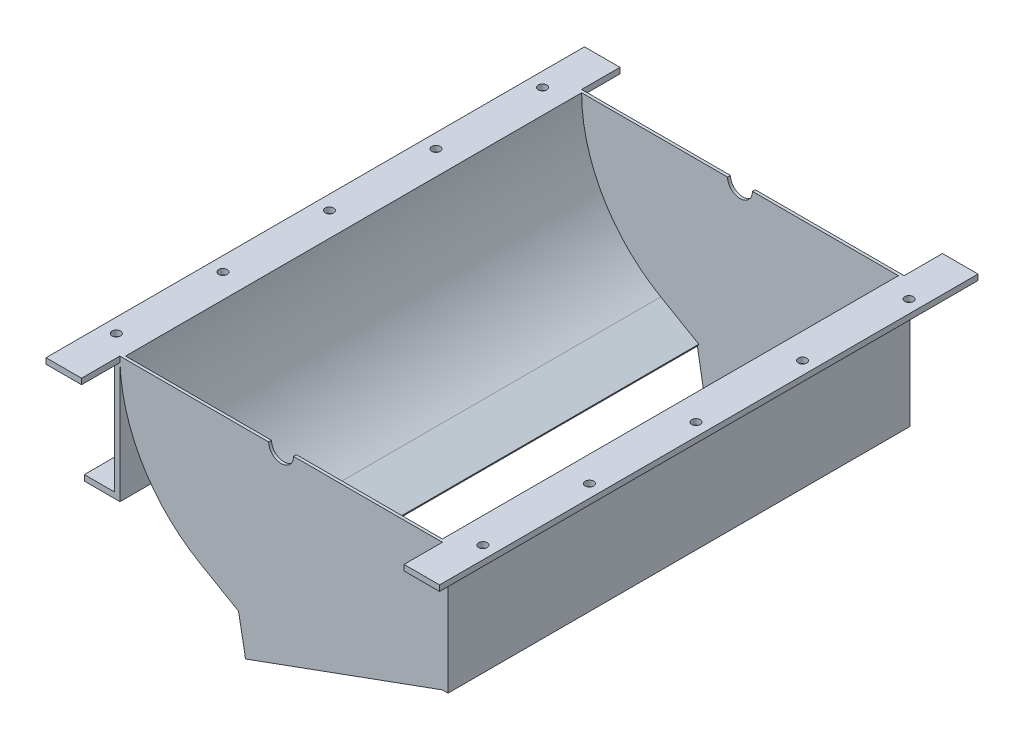
SolidWorks part; units mm, degrees
material "AISI 304"
ref_plane "Front Plane" through (0, 0, 0) normal (0, 0, 1) x (1, 0, 0)
ref_plane "Top Plane" through (0, 0, 0) normal (0, 1, 0) x (1, 0, 0)
ref_plane "Right Plane" through (0, 0, 0) normal (1, 0, 0) x (0, 0, -1)
other "Configuration Table"
sketch "Sketch1" plane through (0, 0, 0) normal (0, 0, 1) x (1, 0, 0)
  line L0 (-227, 0) -> (-227, 377)
  line L1 (-227, 377) -> (0, 377)
  line L2 (0, 377) -> (0, 227)
  line L3 (-223, 0) -> (-223, 377)
  line L4 (-3, 377) -> (-3, 226.9802)
  line L5 (-227, 0) -> (227, 0) construction
  line L7 (227, -180) -> (-50, -280.8198)
  line L8 (223, 0) -> (223, -177.1992)
  line L9 (223, -177.1992) -> (-51.3681, -277.061)
  line L10 (-51.3681, -277.061) -> (-50, -280.8198)
  line L11 (-113.5, -196.5878) -> (-60, -227.476)
  line L12 (-111.5, -193.1237) -> (-58, -224.0119)
  line L13 (-58, -224.0119) -> (-60, -227.476)
  line L14 (-227, 0) -> (-277, 0) construction
  line L15 (227, 0) -> (277, 0) construction
  line L16 (-50, -280.8198) -> (330.4492, -280.8198) construction
  line L17 (-277, 0) -> (-223, 0)
  line L18 (-277, 0) -> (-277, 6)
  line L19 (-277, 6) -> (-223, 6)
  line L20 (-223, 0) -> (-223, 6)
  line L21 (277, 0) -> (226.9207, 0)
  line L22 (277, 0) -> (277, 6)
  line L23 (277, 6) -> (226.9207, 6)
  line L24 (226.9207, 0) -> (226.9207, 6)
  line L25 (-277, 0) -> (-226.859, 0)
  line L26 (-277, 0) -> (-277, -8)
  line L27 (-277, -8) -> (-234.859, -8)
  line L29 (277, 0) -> (223, 0)
  line L30 (277, 0) -> (277, -8)
  line L31 (277, -8) -> (235, -8)
  line L32 (223, 0) -> (223, -8)
  line L34 (-226.859, -8) -> (-226.859, -227.476)
  line L35 (-226.859, -227.476) -> (-234.859, -227.476)
  line L36 (-234.859, -8) -> (-234.859, -219.476)
  line L38 (235, -8) -> (235, -219.476)
  line L39 (235, -227.476) -> (227, -227.476)
  line L40 (227, -180) -> (227, -227.476)
  line L41 (-60, -227.476) -> (-291.314, -227.476) construction
  line L42 (-60, -227.476) -> (-226.859, -227.476)
  line L43 (235, -227.476) -> (279, -227.476)
  line L45 (235, -219.476) -> (279, -219.476)
  line L46 (279, -227.476) -> (279, -219.476)
  line L47 (-234.859, -227.476) -> (-278.859, -227.476)
  line L49 (-234.859, -219.476) -> (-278.859, -219.476)
  line L50 (-278.859, -227.476) -> (-278.859, -219.476)
  line L51 (227, -8) -> (226.859, -8)
  line L52 (227, 0) -> (227, -180) construction
  circle A0 centre (0, 0) radius 208
  circle A1 centre (0, 0) radius 223
  arc A2 (-226.859, -8) -> (223, -42.4264) centre (0, 0) ccw
  circle A3 centre (0, 0) radius 227 construction
  arc A4 (227, 0) -> (-227, 0) centre (0, 0) ccw
  dimension "D1" = 416
  dimension "D4" = 150
  dimension "D5" = 3
  dimension "D6" = 180
  dimension "D8" = 50
  dimension "D10" = 30
  dimension "D11" = 60
  dimension "D12" = 4
  dimension "D13" = 50
  dimension "D14" = 50
  dimension "D15" = 6
  dimension "D16" = 6
  dimension "D17" = 8
  dimension "D18" = 8
  dimension "D19" = 8
  dimension "D20" = 8
  dimension "D21" = 0
  dimension "D22" = 0
  dimension "D23" = 44
  dimension "D24" = 8
  dimension "D25" = 8
  dimension "D26" = 44
  dimension "D2" = 15
  dimension "D3" = 4
  dimension "D9" = 4
extrude "Boss-Extrude2" add sketch "Sketch1" along normal mid plane 650
sketch "Sketch3" plane through (0, 0, 325) normal (0, 0, 1) x (1, 0, 0)
  line L0 (-226.859, -227.476) -> (-226.859, -8) construction
  line L1 (-113.5, -196.5878) -> (-60, -227.476) construction
  line L2 (-60, -227.476) -> (-58, -224.0119) construction
  line L3 (-58, -224.0119) -> (-111.5, -193.1237) construction
  line L4 (-223, 0) -> (-277, 0) construction
  line L5 (-277, 0) -> (-277, -8) construction
  line L6 (-277, -8) -> (-234.859, -8) construction
  line L7 (-234.859, -8) -> (-234.859, -219.476) construction
  line L8 (-234.859, -219.476) -> (-278.859, -219.476) construction
  line L9 (-278.859, -219.476) -> (-278.859, -227.476) construction
  line L10 (-278.859, -227.476) -> (-226.859, -227.476) construction
  line L11 (227, -227.476) -> (279, -227.476) construction
  line L12 (279, -227.476) -> (279, -219.476) construction
  line L13 (279, -219.476) -> (235, -219.476) construction
  line L14 (235, -219.476) -> (235, -8) construction
  line L15 (235, -8) -> (277, -8) construction
  line L16 (277, -8) -> (277, 0) construction
  line L17 (277, 0) -> (223, 0) construction
  line L18 (223, 0) -> (223, -177.1992) construction
  line L19 (223, -177.1992) -> (-51.3681, -277.061) construction
  line L20 (-51.3681, -277.061) -> (-50, -280.8198) construction
  line L21 (-50, -280.8198) -> (227, -180) construction
  line L22 (227, -180) -> (227, -227.476) construction
  line L23 (-226.859, -227.476) -> (-226.859, -8)
  line L24 (-113.5, -196.5878) -> (-60, -227.476)
  line L25 (-60, -227.476) -> (-58, -224.0119)
  line L26 (-58, -224.0119) -> (-111.5, -193.1237)
  line L27 (-223, 0) -> (-277, 0)
  line L28 (-277, 0) -> (-277, -8)
  line L29 (-277, -8) -> (-234.859, -8)
  line L30 (-234.859, -8) -> (-234.859, -219.476)
  line L31 (-234.859, -219.476) -> (-278.859, -219.476)
  line L32 (-278.859, -219.476) -> (-278.859, -227.476)
  line L33 (-278.859, -227.476) -> (-226.859, -227.476)
  line L34 (227, -227.476) -> (279, -227.476)
  line L35 (279, -227.476) -> (279, -219.476)
  line L36 (279, -219.476) -> (235, -219.476)
  line L37 (235, -219.476) -> (235, -8)
  line L38 (235, -8) -> (277, -8)
  line L39 (277, -8) -> (277, 0)
  line L40 (277, 0) -> (223, 0)
  line L41 (223, 0) -> (223, -177.1992)
  line L42 (223, -177.1992) -> (-51.3681, -277.061)
  line L43 (-51.3681, -277.061) -> (-50, -280.8198)
  line L44 (-50, -280.8198) -> (227, -180)
  line L45 (227, -180) -> (227, -227.476)
  line L46 (-60, -227.476) -> (-50, -280.8198)
  line L47 (-226.859, -227.476) -> (227, -227.476)
  line L48 (-223, 0) -> (223, 0)
  arc A0 (-226.859, -8) -> (-113.5, -196.5878) centre (0, 0) ccw construction
  arc A1 (-223, 0) -> (-111.5, -193.1237) centre (0, 0) ccw construction
  arc A2 (-226.859, -8) -> (-113.5, -196.5878) centre (0, 0) ccw
  arc A3 (-223, 0) -> (-111.5, -193.1237) centre (0, 0) ccw
  line M8 (223, 0) -> (223, -177.1992)
  line M9 (223, -177.1992) -> (-51.3681, -277.061)
extrude "Boss-Extrude3" add sketch "Sketch3" against normal blind 4 contours L48 A3 L26 L25 L47 M9 M8 | L47 L46 L42
sketch "Sketch4" plane through (0, 0, -325) normal (0, 0, -1) x (-1, 0, 0)
  line L0 (226.859, -8) -> (226.859, -227.476) construction
  line L1 (226.859, -227.476) -> (278.859, -227.476) construction
  line L2 (278.859, -227.476) -> (278.859, -219.476) construction
  line L3 (278.859, -219.476) -> (234.859, -219.476) construction
  line L4 (234.859, -219.476) -> (234.859, -8) construction
  line L5 (234.859, -8) -> (277, -8) construction
  line L6 (277, -8) -> (277, 0) construction
  line L7 (277, 0) -> (223, 0) construction
  line L8 (111.5, -193.1237) -> (58, -224.0119) construction
  line L9 (58, -224.0119) -> (60, -227.476) construction
  line L10 (60, -227.476) -> (113.5, -196.5878) construction
  line L11 (-279, -227.476) -> (-227, -227.476) construction
  line L12 (-227, -227.476) -> (-227, -180) construction
  line L13 (-227, -180) -> (50, -280.8198) construction
  line L14 (50, -280.8198) -> (51.3681, -277.061) construction
  line L15 (51.3681, -277.061) -> (-223, -177.1992) construction
  line L16 (-223, -177.1992) -> (-223, 0) construction
  line L17 (-223, 0) -> (-277, 0) construction
  line L18 (-277, 0) -> (-277, -8) construction
  line L19 (-277, -8) -> (-235, -8) construction
  line L20 (-235, -8) -> (-235, -219.476) construction
  line L21 (-235, -219.476) -> (-279, -219.476) construction
  line L22 (-279, -219.476) -> (-279, -227.476) construction
  line L23 (226.859, -8) -> (226.859, -227.476)
  line L24 (226.859, -227.476) -> (278.859, -227.476)
  line L25 (278.859, -227.476) -> (278.859, -219.476)
  line L26 (278.859, -219.476) -> (234.859, -219.476)
  line L27 (234.859, -219.476) -> (234.859, -8)
  line L28 (234.859, -8) -> (277, -8)
  line L29 (277, -8) -> (277, 0)
  line L30 (277, 0) -> (223, 0)
  line L31 (111.5, -193.1237) -> (58, -224.0119)
  line L32 (58, -224.0119) -> (60, -227.476)
  line L33 (60, -227.476) -> (113.5, -196.5878)
  line L34 (-279, -227.476) -> (-227, -227.476)
  line L35 (-227, -227.476) -> (-227, -180)
  line L36 (-227, -180) -> (50, -280.8198)
  line L37 (50, -280.8198) -> (51.3681, -277.061)
  line L38 (51.3681, -277.061) -> (-223, -177.1992)
  line L39 (-223, -177.1992) -> (-223, 0)
  line L40 (-223, 0) -> (-277, 0)
  line L41 (-277, 0) -> (-277, -8)
  line L42 (-277, -8) -> (-235, -8)
  line L43 (-235, -8) -> (-235, -219.476)
  line L44 (-235, -219.476) -> (-279, -219.476)
  line L45 (-279, -219.476) -> (-279, -227.476)
  line L46 (-223, 0) -> (223, 0)
  line L47 (60, -227.476) -> (51.3681, -277.061)
  arc A0 (111.5, -193.1237) -> (223, 0) centre (0, 0) ccw construction
  arc A1 (113.5, -196.5878) -> (226.859, -8) centre (0, 0) ccw construction
  arc A2 (111.5, -193.1237) -> (223, 0) centre (0, 0) ccw
  arc A3 (113.5, -196.5878) -> (226.859, -8) centre (0, 0) ccw
  line M5 (51.3681, -277.061) -> (-223, -177.1992)
  line M6 (-223, -177.1992) -> (-223, 0)
extrude "Boss-Extrude4" add sketch "Sketch4" against normal blind 4 contours L31 A2 L46 L47 L32 M6 M5
sketch "Sketch5" plane through (0, 0, 0) normal (0, 1, 0) x (1, 0, 0)
  line L0 (-257, 325) -> (-257, -325) construction
  line L1 (277, 325) -> (-277, 325) construction
  line L2 (277, -325) -> (-277, -325) construction
  line L3 (-277, -325) -> (-277, 325) construction
  line L4 (259, 325) -> (259, -325) construction
  line L5 (279, -325) -> (279, 325) construction
  circle A0 centre (-257, 0) radius 6
  circle A1 centre (259, 0) radius 6
  dimension "D3" = 12
  dimension "D4" = 12
  dimension "D1" = 20
  dimension "D2" = 20
extrude "Cut-Extrude1" cut sketch "Sketch5" against normal blind 10
pattern_linear "LPattern1" count 3 spacing 150 along (0, 0, -1) of "Cut-Extrude1"
pattern_linear "LPattern2" count 3 spacing 150 along (0, 0, 1) of "LPattern1"
sketch "Sketch6" plane through (0, 0, -325) normal (0, 0, -1) x (-1, 0, 0)
  circle A0 centre (0, 0) radius 17.5
  dimension "D1" = 35
extrude "Cut-Extrude2" cut sketch "Sketch6" against normal through all both and the other way through all
sketch "Sketch7" plane through (0, 0, 325) normal (0, 0, 1) x (1, 0, 0)
  line L1 (-226.859, -227.476) -> (-327.2292, -227.476)
  line L2 (-226.859, -227.476) -> (-226.859, -177.476)
  line L3 (-226.859, -177.476) -> (-327.2292, -177.476)
  line L4 (-327.2292, -227.476) -> (-327.2292, -177.476)
  dimension "D1" = 50
extrude "Cut-Extrude3" cut sketch "Sketch7" against normal through all both and the other way through all
sketch "Sketch8" plane through (-234.859, 0, 0) normal (-1, 0, 0) x (0, 0, 1)
  line L0 (-325, -8) -> (-325, -177.476) construction
  line L1 (325, -177.476) -> (-325, -177.476)
  line L2 (325, -177.476) -> (325, -169.476)
  line L3 (325, -169.476) -> (-325, -169.476)
  line L4 (-325, -177.476) -> (-325, -169.476)
  dimension "D1" = 8
extrude "Boss-Extrude5" add sketch "Sketch8" along normal up to surface (42.141 mm away) up to face at (-277, -4, 0)
sketch "Sketch9" plane through (0, 0, 325) normal (0, 0, 1) x (1, 0, 0)
  line L3 (227, -180) -> (326.0243, -180)
  line L4 (227, -180) -> (227, -265.7989)
  line L5 (227, -265.7989) -> (326.0243, -265.7989)
  line L6 (326.0243, -180) -> (326.0243, -265.7989)
extrude "Cut-Extrude4" cut sketch "Sketch9" against normal through all both and the other way through all
sketch "Sketch10" plane through (0, 0, 0) normal (0, 1, 0) x (1, 0, 0)
  line L1 (-277, 325) -> (-227, 325)
  line L2 (-277, 325) -> (-277, 379)
  line L3 (-277, 379) -> (-227, 379)
  line L4 (-227, 325) -> (-227, 379)
  line L5 (277, 325) -> (227, 325)
  line L6 (277, 325) -> (277, 379)
  line L7 (277, 379) -> (227, 379)
  line L8 (227, 325) -> (227, 379)
  line L9 (277, -325) -> (227, -325)
  line L10 (277, -325) -> (277, -379)
  line L11 (277, -379) -> (227, -379)
  line L12 (227, -325) -> (227, -379)
  line L13 (-277, -325) -> (-227, -325)
  line L14 (-277, -325) -> (-277, -379)
  line L15 (-277, -379) -> (-227, -379)
  line L16 (-227, -325) -> (-227, -379)
  dimension "D1" = 50
  dimension "D2" = 50
  dimension "D3" = 50
  dimension "D4" = 50
  dimension "D5" = 54
  dimension "D6" = 54
  dimension "D7" = 54
  dimension "D8" = 54
extrude "Boss-Extrude6" add sketch "Sketch10" against normal up to surface (8 mm away) up to face at (-263, -8, 300)
